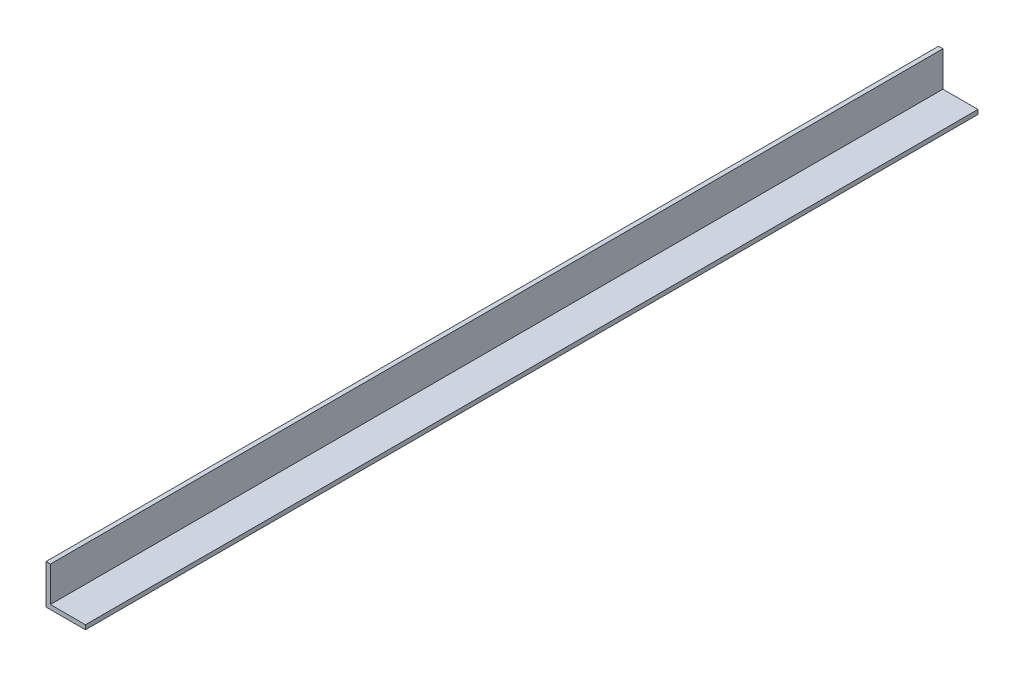
SolidWorks part; units mm, degrees
material "1023 碳钢板 (SS)"
ref_plane "Front Plane" through (0, 0, 0) normal (0, 0, 1) x (1, 0, 0)
ref_plane "Top Plane" through (0, 0, 0) normal (0, 1, 0) x (1, 0, 0)
ref_plane "Right Plane" through (0, 0, 0) normal (1, 0, 0) x (0, 0, -1)
sketch "Sketch1" plane through (0, 0, 0) normal (0, 0, 1) x (1, 0, 0)
  line L0 (-46.7067, 40) -> (-46.7067, -5)
  line L1 (-46.7067, -5) -> (-1.7067, -5)
  line L2 (-1.7067, -5) -> (-1.7067, 0)
  line L3 (-1.7067, 0) -> (-41.7067, 0)
  line L4 (-41.7067, 0) -> (-41.7067, 40)
  line L5 (-41.7067, 40) -> (-46.7067, 40)
  dimension "D1" = 5
  dimension "D2" = 5
  dimension "D3" = 45
  dimension "D4" = 45
extrude "Extrude1" add sketch "Sketch1" along normal blind 1018.7
